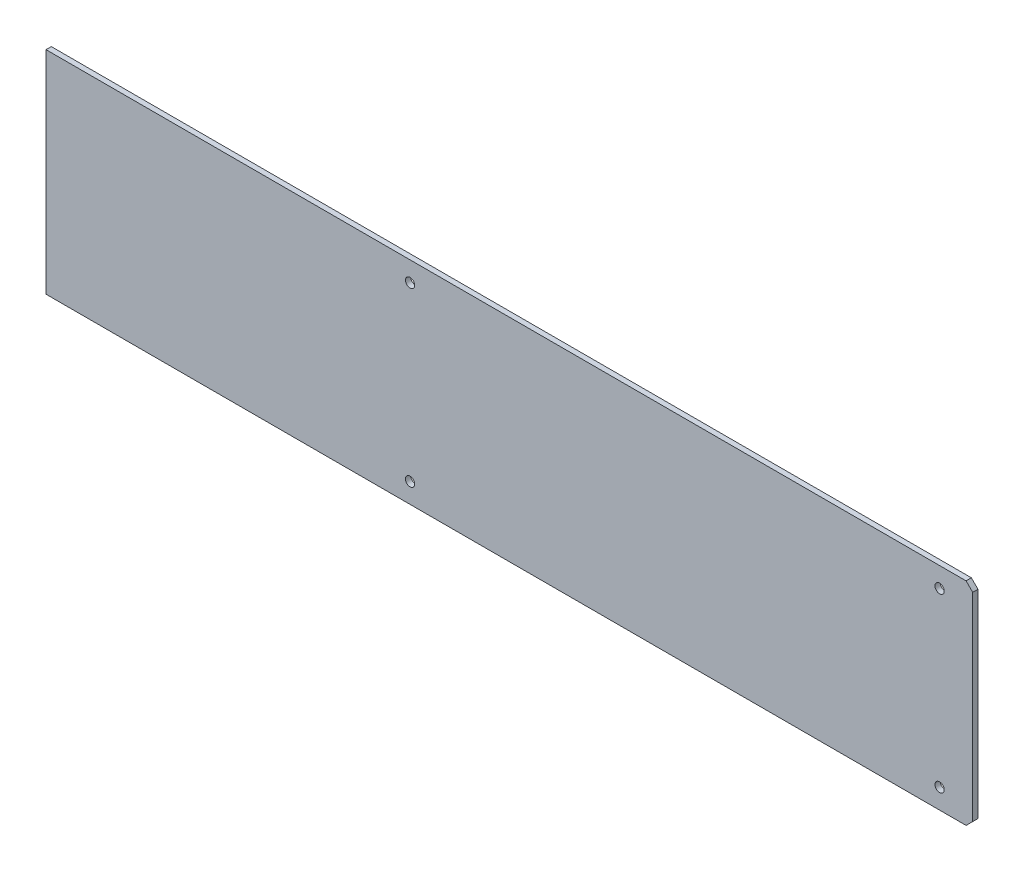
SolidWorks part; units mm, degrees
material "1023 carbon steel plate (SS)"
ref_plane "Front Plane" through (0, 0, 0) normal (0, 0, 1) x (1, 0, 0)
ref_plane "Top Plane" through (0, 0, 0) normal (0, 1, 0) x (1, 0, 0)
ref_plane "Right Plane" through (0, 0, 0) normal (1, 0, 0) x (0, 0, -1)
sketch "Sketch1" plane through (0, 0, 0) normal (0, 0, 1) x (1, 0, 0)
  line L1 (-350, 80) -> (350, 80)
  line L2 (-350, 80) -> (-350, -80)
  line L3 (-350, -80) -> (350, -80)
  line L4 (350, 80) -> (350, -80)
  line L5 (-350, 80) -> (350, -80) construction
  line L6 (-350, -80) -> (350, 80) construction
  point P0 (0, 0)
  dimension "D1" = 700
  dimension "D2" = 160
extrude "Boss-Extrude1" add sketch "Sketch1" along normal blind 4 contours L2 L1 L4 L3
sketch "Sketch2" plane through (0, 0, 4) normal (0, 0, 1) x (1, 0, 0)
  line L0 (-350, 80) -> (350, 80) construction
  line L1 (350, 80) -> (350, -80) construction
  circle A0 centre (-75, 65) radius 3.5
  circle A1 centre (325, 65) radius 3.5
  circle A2 centre (325, -65) radius 3.5
  circle A3 centre (-75, -65) radius 3.5
  dimension "D5" = 7
  dimension "D1" = 400
  dimension "D2" = 130
  dimension "D3" = 15
  dimension "D4" = 25
extrude "Cut-Extrude1" cut sketch "Sketch2" against normal blind 4
chamfer "Chamfer1" distance 5 angle 45 2 edges at (350, -80, 2) (350, 80, 2)
